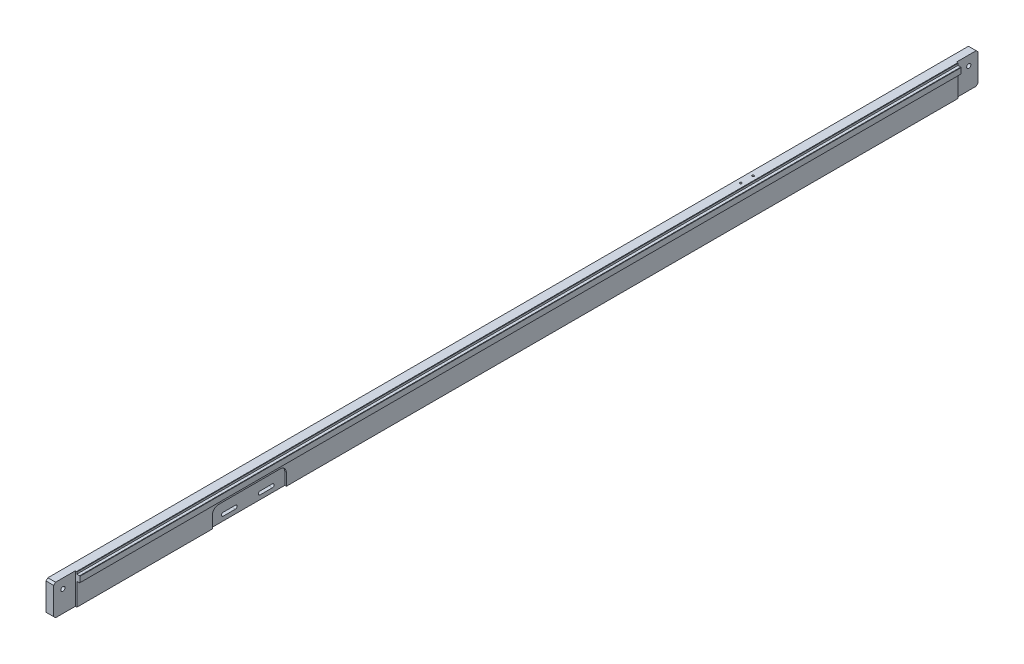
from build123d import *

# Parameters (mm, degrees)
SKETCH_1_W             = 1430
SKETCH_1_H             = 50
EXTRUDE_1_DEPTH        = 15
SKETCH_5_W             = 1430
SKETCH_5_H             = 10
EXTRUDE_3_DEPTH        = 5
HOLE_WIZARD_M6_2_D     = 5
HOLE_WIZARD_M6_2_DEPTH = 17
HOLE_WIZARD_M6_2_TIP   = 1.502151548
CHAMFER_2_SIZE         = 0.5
SKETCH_10_W            = 35
SKETCH_10_H            = 50
EXTRUDE_4_DEPTH        = 12.5
HOLE_WIZARD_M8_1_D     = 6.8
CHAMFER_3_SIZE         = 3
CUT_EXTRUDE_1_DEPTH    = 751.68302232
SKETCH_14_W            = 120
SKETCH_14_H            = 29.5
CUT_EXTRUDE_2_DEPTH    = 2.5
FILLET_1_R             = 10
HOLE_WIZARD_M6_3_D     = 5
HOLE_WIZARD_M6_3_DEPTH = 17
HOLE_WIZARD_M6_3_TIP   = 1.502151548
HOLE_WIZARD_M6_5_D     = 5
HOLE_WIZARD_M6_5_DEPTH = 17
HOLE_WIZARD_M6_5_TIP   = 1.502151548
HOLE_WIZARD_M4_1_D     = 3.3
HOLE_WIZARD_M4_1_DEPTH = 11.5
HOLE_WIZARD_M4_1_TIP   = 0.991420021
HOLE_WIZARD_M4_2_D     = 3.3
HOLE_WIZARD_M4_2_DEPTH = 11.5
HOLE_WIZARD_M4_2_TIP   = 0.991420021
HOLE_WIZARD_M4_3_D     = 3.3
HOLE_WIZARD_M4_3_DEPTH = 11.5
HOLE_WIZARD_M4_3_TIP   = 0.991420021


with BuildPart() as part:
    # 草图1 → 凸台-拉伸1 (new body)
    with BuildSketch(Plane(origin=(0, 0, 0), x_dir=(0, 0, -1), z_dir=(1, 0, 0))):
        Rectangle(SKETCH_1_W, SKETCH_1_H)
    extrude(amount=EXTRUDE_1_DEPTH)

    # 草图5 → 凸台-拉伸3 (add)
    with BuildSketch(Plane(origin=(15, 0, 0), x_dir=(0, 0, -1), z_dir=(1, 0, 0))):
        with Locations((0, 16.5)):
            Rectangle(SKETCH_5_W, SKETCH_5_H)
    extrude(amount=EXTRUDE_3_DEPTH)

    # M6 螺纹孔2
    with Locations(Plane(origin=(-9.706715775, -25, 33.268833901), x_dir=(0, 0, -1), z_dir=(0, -1, 0))):
        with Locations((-581.731166099, 17.206715775), (-536.731166099, 17.206715775), (323.268833901, 17.206715775), (278.268833901, 17.206715775)):
            Hole(HOLE_WIZARD_M6_2_D / 2, depth=HOLE_WIZARD_M6_2_DEPTH)
            with Locations((0, 0, -(HOLE_WIZARD_M6_2_DEPTH + HOLE_WIZARD_M6_2_TIP / 2))):  # 118° drill point
                Cone(0, HOLE_WIZARD_M6_2_D / 2, HOLE_WIZARD_M6_2_TIP, mode=Mode.SUBTRACT)

    # 倒角2
    chamfer_2_edges = [part.edges().sort_by_distance(p)[0] for p in [
        (15, 25, 0),
        (20, 21.5, 0),
        (20, 11.5, 0),
    ]]
    chamfer(chamfer_2_edges, length=CHAMFER_2_SIZE)

    # 草图10 → 凸台-拉伸4 (add)
    with BuildSketch(Plane.ZY):
        with Locations((-732.5, 0)):
            Rectangle(SKETCH_10_W, SKETCH_10_H)
        with Locations((732.5, 0)):
            Rectangle(SKETCH_10_W, SKETCH_10_H)
    extrude(amount=-EXTRUDE_4_DEPTH)

    # M8 螺纹孔1 (through all)
    with Locations(Plane(origin=(12.5, 0, 0), x_dir=(0, 0, -1), z_dir=(1, 0, 0))):
        with Locations((-735, 9.5), (735, 9.5)):
            Hole(HOLE_WIZARD_M8_1_D / 2)

    # 倒角3
    chamfer_3_edges = [part.edges().sort_by_distance(p)[0] for p in [
        (6.25, -25, -750),
        (6.25, 25, -750),
        (6.25, -25, 750),
        (6.25, 25, 750),
    ]]
    chamfer(chamfer_3_edges, length=CHAMFER_3_SIZE)

    # 草图13 → 切除-拉伸1 (cut, through all)
    with BuildSketch(Plane.ZY):
        with BuildLine():
            Line((395, -12.75), (415, -12.75))
            ThreePointArc((415, -12.75), (417.75, -15.5), (415, -18.25))
            Line((415, -18.25), (395, -18.25))
            ThreePointArc((395, -18.25), (392.25, -15.5), (395, -12.75))
        make_face()
        with BuildLine():
            Line((455, -12.75), (475, -12.75))
            ThreePointArc((475, -12.75), (477.75, -15.5), (475, -18.25))
            Line((475, -18.25), (455, -18.25))
            ThreePointArc((455, -18.25), (452.25, -15.5), (455, -12.75))
        make_face()
    extrude(amount=-CUT_EXTRUDE_1_DEPTH, mode=Mode.SUBTRACT)

    # 草图14 → 切除-拉伸2 (cut)
    with BuildSketch(Plane(origin=(15, 0, 0), x_dir=(0, 0, -1), z_dir=(1, 0, 0))):
        with Locations((-435, -10.25)):
            Rectangle(SKETCH_14_W, SKETCH_14_H)
    extrude(amount=-CUT_EXTRUDE_2_DEPTH, mode=Mode.SUBTRACT)

    # 圆角1
    fillet_1_edges = [part.edges().sort_by_distance(p)[0] for p in [
        (13.75, 4.5, 495),
        (13.75, 4.5, 375),
    ]]
    fillet(fillet_1_edges, radius=FILLET_1_R)

    # M6 螺纹孔3
    with Locations(Plane(origin=(0, -25, 0), x_dir=(-1, 0, 0), z_dir=(0, -1, 0))):
        with Locations((-7.5, 133.512), (-7.5, 158.512)):
            Hole(HOLE_WIZARD_M6_3_D / 2, depth=HOLE_WIZARD_M6_3_DEPTH)
            with Locations((0, 0, -(HOLE_WIZARD_M6_3_DEPTH + HOLE_WIZARD_M6_3_TIP / 2))):  # 118° drill point
                Cone(0, HOLE_WIZARD_M6_3_D / 2, HOLE_WIZARD_M6_3_TIP, mode=Mode.SUBTRACT)

    # M6 螺纹孔5
    with Locations(Plane(origin=(0, -25, 0), x_dir=(-1, 0, 0), z_dir=(0, -1, 0))):
        with Locations((-6.25, -492.5), (-6.25, -387.5)):
            Hole(HOLE_WIZARD_M6_5_D / 2, depth=HOLE_WIZARD_M6_5_DEPTH)
            with Locations((0, 0, -(HOLE_WIZARD_M6_5_DEPTH + HOLE_WIZARD_M6_5_TIP / 2))):  # 118° drill point
                Cone(0, HOLE_WIZARD_M6_5_D / 2, HOLE_WIZARD_M6_5_TIP, mode=Mode.SUBTRACT)

    # M4 螺纹孔1
    with Locations(Plane(origin=(0, 0, -750), x_dir=(-1, 0, 0), z_dir=(0, 0, -1))):
        with Locations((-6.25, 15), (-6.25, 0)):
            Hole(HOLE_WIZARD_M4_1_D / 2, depth=HOLE_WIZARD_M4_1_DEPTH)
            with Locations((0, 0, -(HOLE_WIZARD_M4_1_DEPTH + HOLE_WIZARD_M4_1_TIP / 2))):  # 118° drill point
                Cone(0, HOLE_WIZARD_M4_1_D / 2, HOLE_WIZARD_M4_1_TIP, mode=Mode.SUBTRACT)

    # M4 螺纹孔2
    with Locations(Plane(origin=(0, 25, 0), x_dir=(1, 0, 0), z_dir=(0, 1, 0))):
        with Locations((7.5, 390), (7.5, 370)):
            Hole(HOLE_WIZARD_M4_2_D / 2, depth=HOLE_WIZARD_M4_2_DEPTH)
            with Locations((0, 0, -(HOLE_WIZARD_M4_2_DEPTH + HOLE_WIZARD_M4_2_TIP / 2))):  # 118° drill point
                Cone(0, HOLE_WIZARD_M4_2_D / 2, HOLE_WIZARD_M4_2_TIP, mode=Mode.SUBTRACT)

    # M4 螺纹孔3
    with Locations(Plane(origin=(0, -25, 0), x_dir=(-1, 0, 0), z_dir=(0, -1, 0))):
        with Locations((-7.5, 122.012), (-7.5, 102.012), (-7.5, 82.012), (-7.5, 62.012), (-7.5, 42.012)):
            Hole(HOLE_WIZARD_M4_3_D / 2, depth=HOLE_WIZARD_M4_3_DEPTH)
            with Locations((0, 0, -(HOLE_WIZARD_M4_3_DEPTH + HOLE_WIZARD_M4_3_TIP / 2))):  # 118° drill point
                Cone(0, HOLE_WIZARD_M4_3_D / 2, HOLE_WIZARD_M4_3_TIP, mode=Mode.SUBTRACT)


solid = part.part
